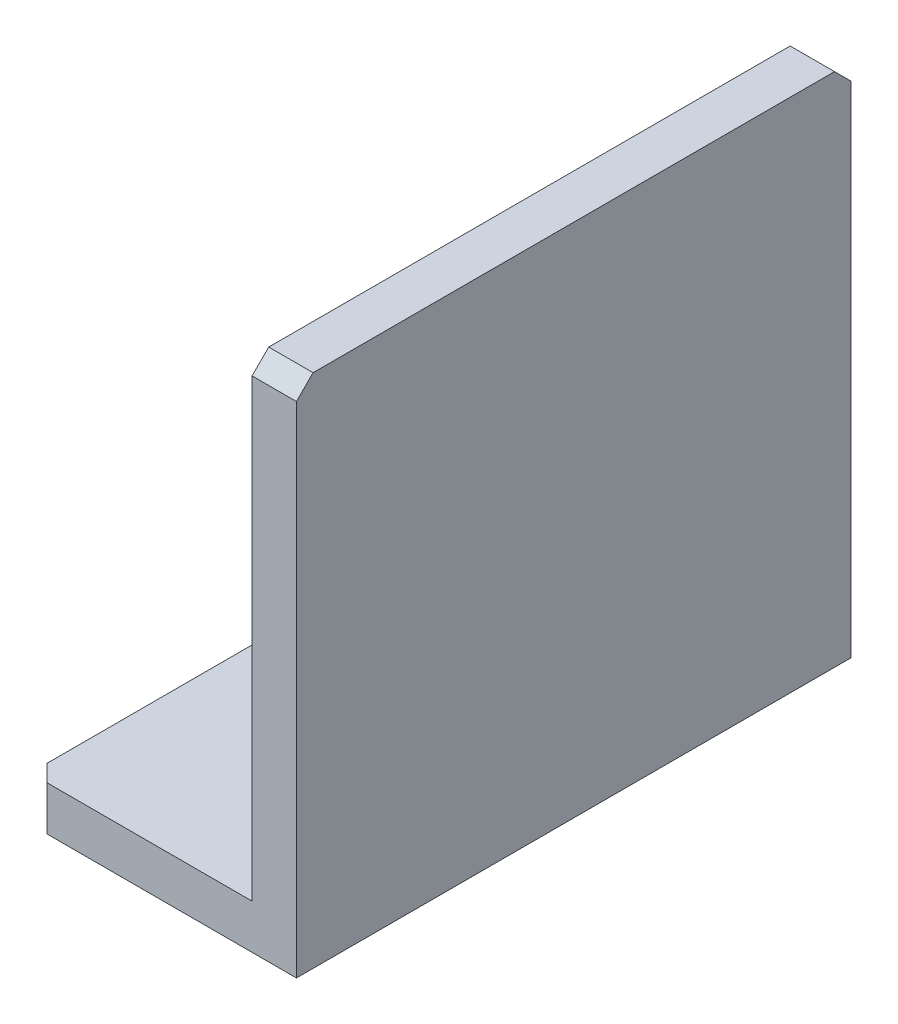
SolidWorks part; units mm, degrees
ref_plane "前视基准面" through (0, 0, 0) normal (0, 0, 1) x (1, 0, 0)
ref_plane "上视基准面" through (0, 0, 0) normal (0, 1, 0) x (1, 0, 0)
ref_plane "右视基准面" through (0, 0, 0) normal (1, 0, 0) x (0, 0, -1)
sketch "草图2" plane through (409.6376, 0.5, -34.3795) normal (0, 0, 1) x (1, 0, 0)
  line L0 (-409.6376, 92.5) -> (-409.6376, -0.5)
  line L1 (-409.6376, -0.5) -> (-457.6376, -0.5)
  line L2 (-457.6376, -0.5) -> (-457.6376, 7.5)
  line L3 (-457.6376, 7.5) -> (-417.6376, 7.5)
  line L4 (-417.6376, 7.5) -> (-417.6376, 92.5)
  line L5 (-417.6376, 92.5) -> (-409.6376, 92.5)
  dimension "D2" = 8
  dimension "D3" = 8
  dimension "D4" = 85
  dimension "D5" = 40
extrude "凸台-拉伸1" add sketch "草图2" along normal mid plane 100
chamfer "倒角1" distance 3 angle 45
